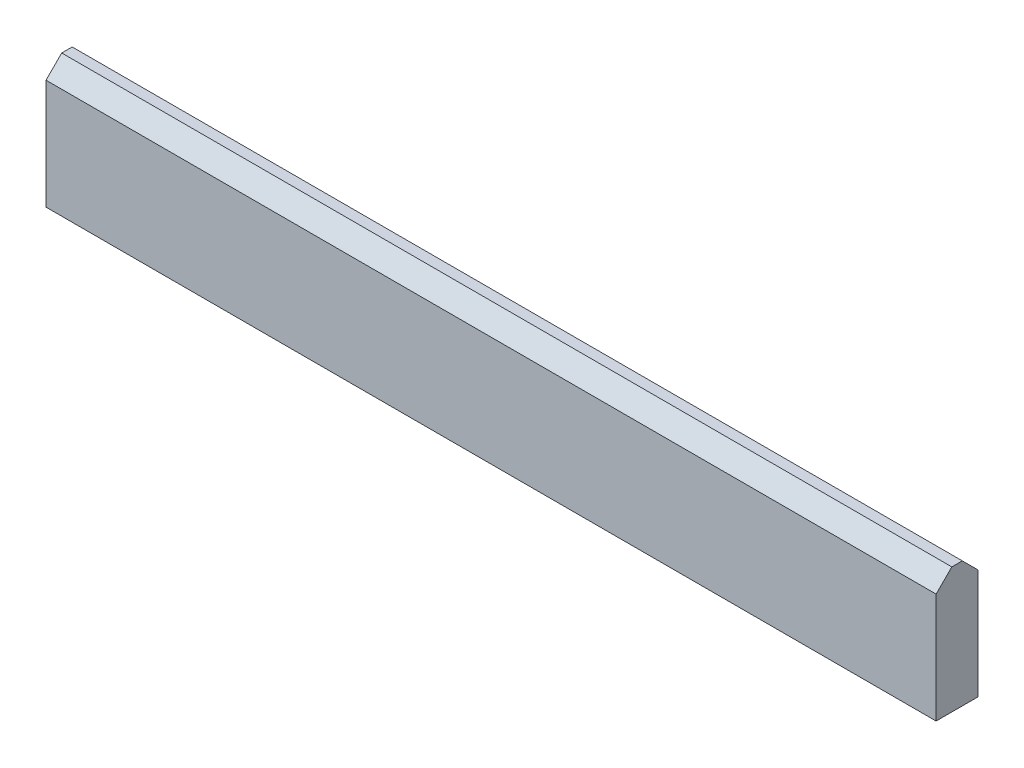
SolidWorks part; units mm, degrees
material "Q235-A"
ref_plane "Front Plane" through (0, 0, 0) normal (0, 0, 1) x (1, 0, 0)
ref_plane "Top Plane" through (0, 0, 0) normal (0, 1, 0) x (1, 0, 0)
ref_plane "Right Plane" through (0, 0, 0) normal (1, 0, 0) x (0, 0, -1)
sketch "Sketch1" plane through (0, 0, 0) normal (0, 0, 1) x (1, 0, 0)
  line L1 (425, -60) -> (-425, -60)
  line L2 (425, -60) -> (425, 60)
  line L3 (425, 60) -> (-425, 60)
  line L4 (-425, -60) -> (-425, 60)
  line L5 (425, -60) -> (-425, 60) construction
  line L6 (425, 60) -> (-425, -60) construction
  point P0 (0, 0)
  dimension "D1" = 850
  dimension "D2" = 120
extrude "Boss-Extrude1" add sketch "Sketch1" along normal mid plane 40
chamfer "Chamfer1" distance 15 angle 45 2 edges at (0, 60, -20) (0, 60, 20)
